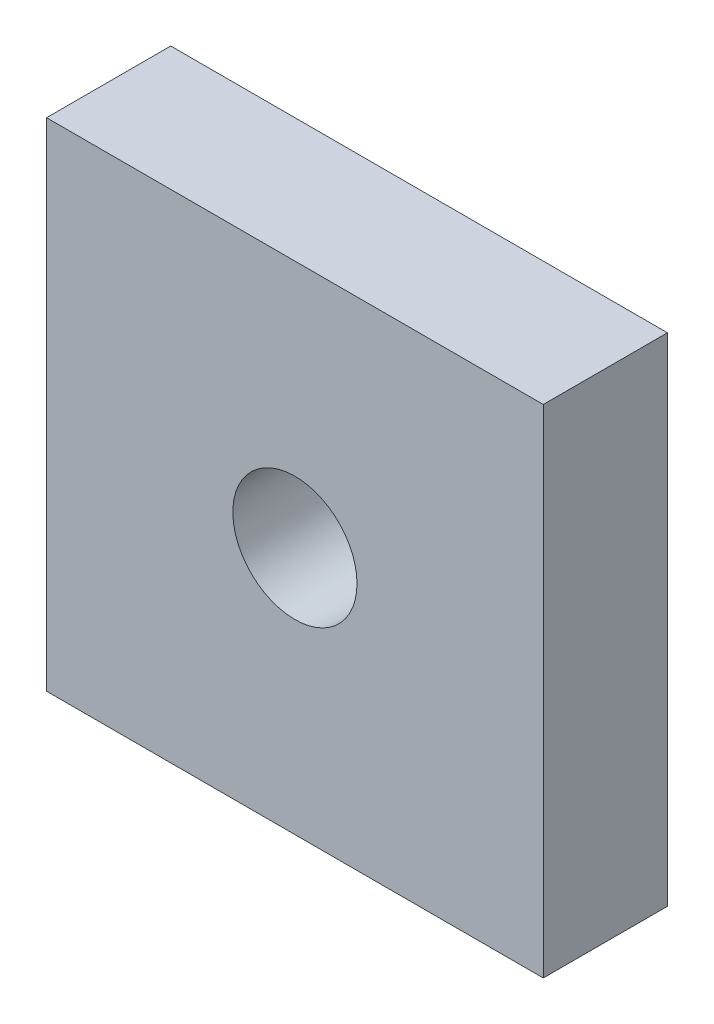
from build123d import *

# Parameters (mm, degrees)
SKETCH1_W           = 40
SKETCH1_H           = 40
SKETCH1_R           = 5
BOSS_EXTRUDE1_DEPTH = 10


with BuildPart() as part:
    # Sketch1 → Boss-Extrude1 (new body)
    with BuildSketch(Plane.XY):
        with Locations((20, 20)):
            Rectangle(SKETCH1_W, SKETCH1_H)
        with Locations((20, 20)):
            Circle(SKETCH1_R, mode=Mode.SUBTRACT)
    extrude(amount=BOSS_EXTRUDE1_DEPTH)


solid = part.part
